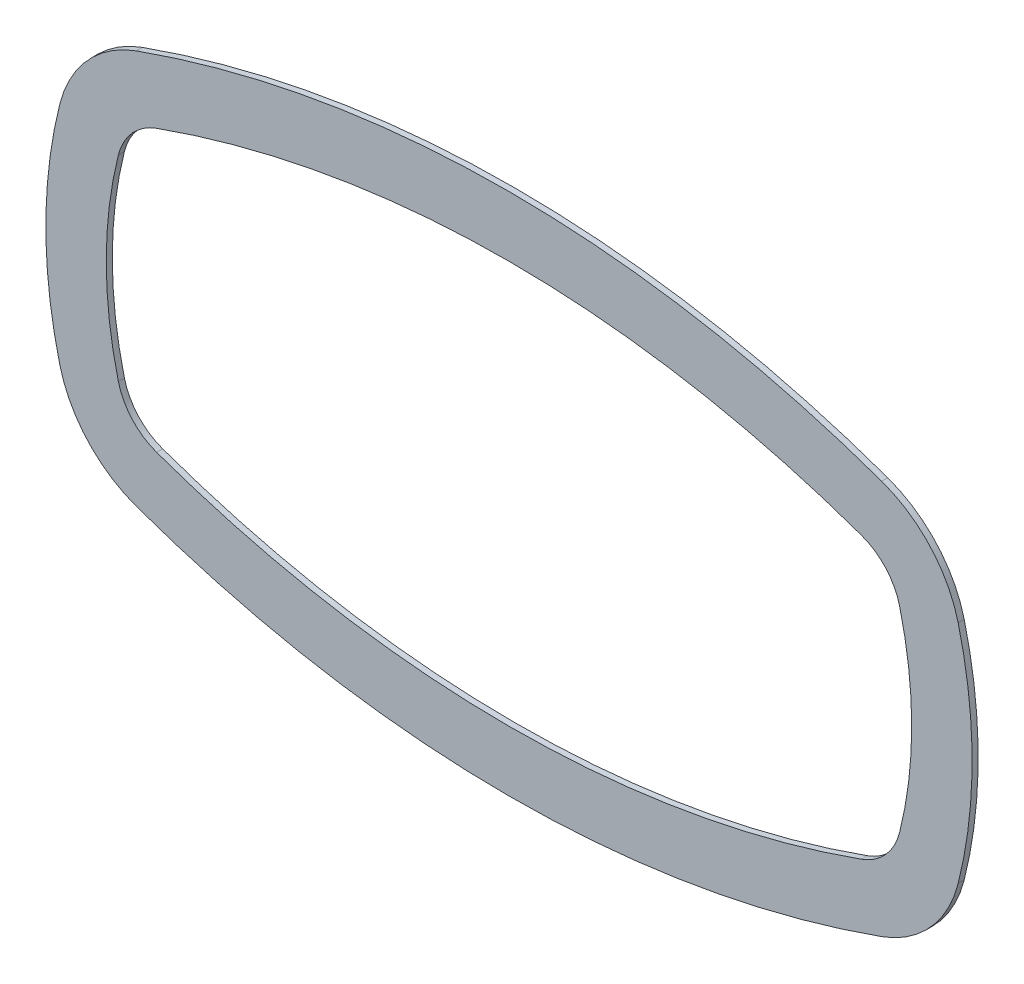
SolidWorks part; units mm, degrees
ref_plane "Front Plane" through (0, 0, 0) normal (0, 0, 1) x (1, 0, 0)
ref_plane "Top Plane" through (0, 0, 0) normal (0, 1, 0) x (1, 0, 0)
ref_plane "Right Plane" through (0, 0, 0) normal (1, 0, 0) x (0, 0, -1)
sketch "Sketch1" plane through (0, 0, 0) normal (0, 0, 1) x (1, 0, 0)
  point P10 (189.3868, -64.2857)
  point P17 (-189.3868, -64.2857)
  point P20 (189.3868, 64.2857)
  point P23 (-189.3868, 64.2857)
  arc B0 (-174.9691, 69.6793) -> (174.9691, 69.6793) centre (0, -420) cw
  arc B1 (-174.9691, -69.6793) -> (174.9691, -69.6793) centre (0, 420) ccw
  arc B2 (193.9703, 48.7395) -> (193.9703, -48.7395) centre (0, 0) cw
  arc B3 (-193.9703, -48.7395) -> (-193.9703, 48.7395) centre (0, 0) cw
  arc B4 (174.9691, -69.6793) -> (193.9703, -48.7395) centre (164.8747, -41.4286) ccw
  arc B5 (-174.9691, -69.6793) -> (-193.9703, -48.7395) centre (-164.8747, -41.4286) cw
  arc B6 (174.9691, 69.6793) -> (193.9703, 48.7395) centre (164.8747, 41.4286) cw
  arc B7 (-174.9691, 69.6793) -> (-193.9703, 48.7395) centre (-164.8747, 41.4286) ccw
  arc B8 (-185.0635, 97.93) -> (185.0635, 97.93) centre (0, -420) cw
  arc B9 (185.0635, 97.93) -> (223.0658, 56.0504) centre (164.8747, 41.4286) cw
  arc B10 (223.0658, 56.0504) -> (223.0658, -56.0504) centre (0, 0) cw
  arc B11 (185.0635, -97.93) -> (223.0658, -56.0504) centre (164.8747, -41.4286) ccw
  arc B12 (-185.0635, -97.93) -> (185.0635, -97.93) centre (0, 420) ccw
  arc B13 (-185.0635, -97.93) -> (-223.0658, -56.0504) centre (-164.8747, -41.4286) cw
  arc B14 (-223.0658, -56.0504) -> (-223.0658, 56.0504) centre (0, 0) cw
  arc B15 (-185.0635, 97.93) -> (-223.0658, 56.0504) centre (-164.8747, 41.4286) ccw
sketch_block_instance "Block1-1-1"
sketch_block "Block1-1" parameters "D1"=520, "D2"=200, "D3"=200, "D4"=30, "D5"=200, "D6"=200, "D7"=30
extrude "Boss-Extrude1" add sketch "Sketch1" along normal blind 3
sketch "Sketch2" plane through (0, 0, 3) normal (0, 0, 1) x (1, 0, 0)
  arc B0 (174.9691, 69.6793) -> (-174.9691, 69.6793) centre (0, -420) ccw
  arc B1 (-185.0635, 97.93) -> (-223.0658, 56.0504) centre (-164.8747, 41.4286) ccw
  arc B2 (-223.0658, 56.0504) -> (-223.0658, -56.0504) centre (0, 0) ccw
  arc B3 (-223.0658, -56.0504) -> (-185.0635, -97.93) centre (-164.8747, -41.4286) ccw
  arc B4 (-185.0635, -97.93) -> (185.0635, -97.93) centre (0, 420) ccw
  arc B5 (185.0635, -97.93) -> (223.0658, -56.0504) centre (164.8747, -41.4286) ccw
  arc B6 (223.0658, -56.0504) -> (223.0658, 56.0504) centre (0, 0) ccw
  arc B7 (223.0658, 56.0504) -> (185.0635, 97.93) centre (164.8747, 41.4286) ccw
  arc B8 (185.0635, 97.93) -> (-185.0635, 97.93) centre (0, -420) ccw
  arc B9 (193.9703, -48.7395) -> (193.9703, 48.7395) centre (0, 0) ccw
  arc B10 (174.9691, -69.6793) -> (193.9703, -48.7395) centre (164.8747, -41.4286) ccw
  arc B11 (-174.9691, -69.6793) -> (174.9691, -69.6793) centre (0, 420) ccw
  arc B12 (-193.9703, -48.7395) -> (-174.9691, -69.6793) centre (-164.8747, -41.4286) ccw
  arc B13 (-193.9703, 48.7395) -> (-193.9703, -48.7395) centre (0, 0) ccw
  arc B14 (-174.9691, 69.6793) -> (-193.9703, 48.7395) centre (-164.8747, 41.4286) ccw
  arc B15 (174.9691, 69.6793) -> (-174.9691, 69.6793) centre (0, -420) ccw
  arc B16 (193.9703, 48.7395) -> (174.9691, 69.6793) centre (164.8747, 41.4286) ccw
sketch_block_instance "Block2-1-1"
sketch_block "Block2-1"
